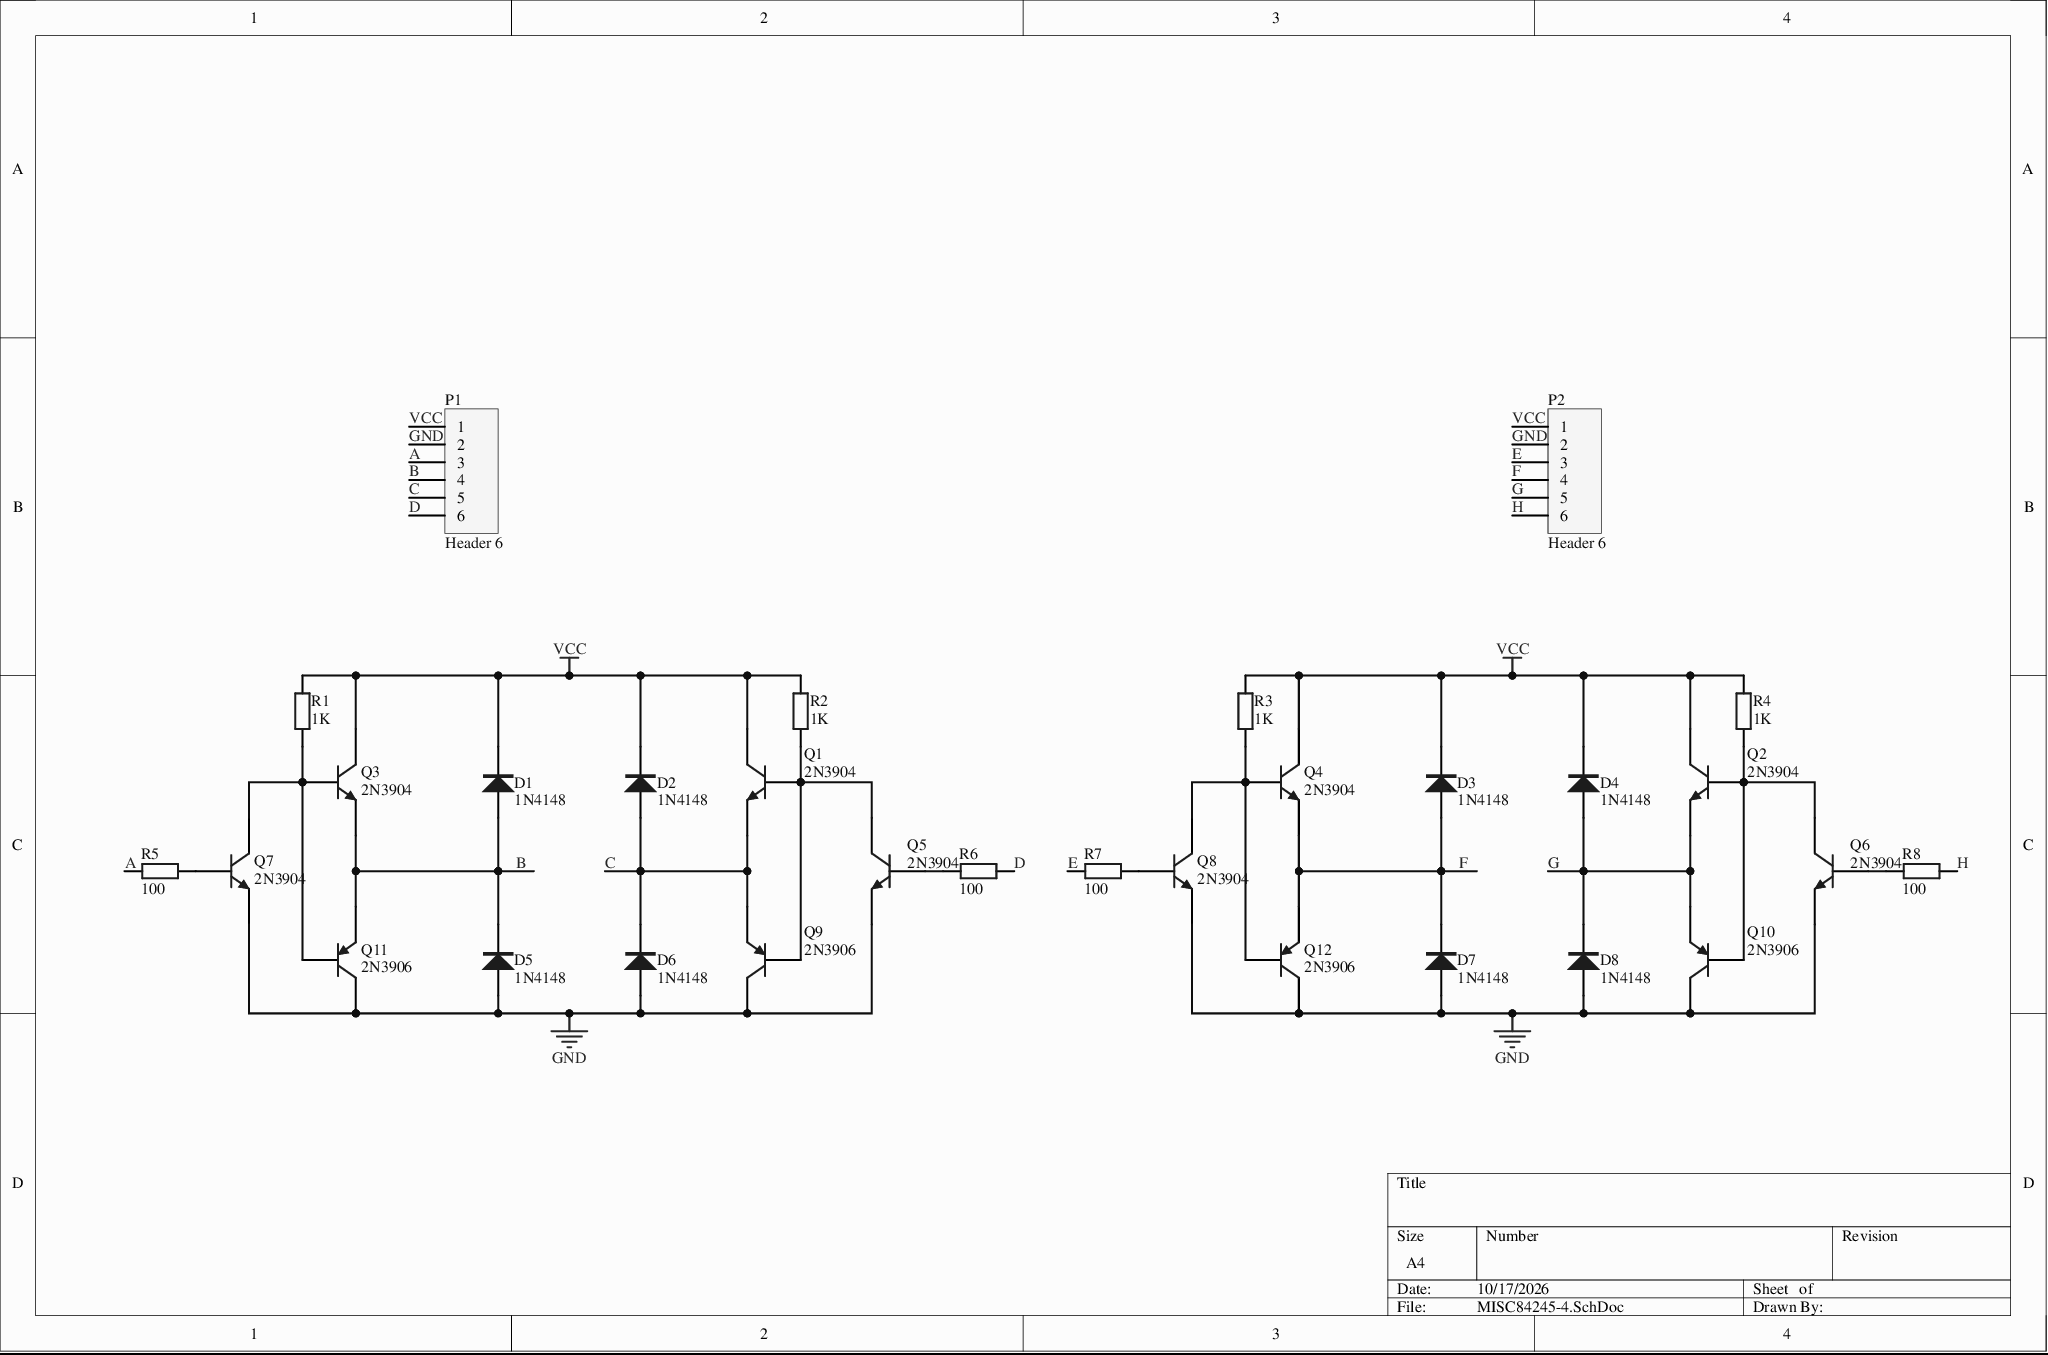
[diagram p0: MISC84245-4.SchDoc]
# Altium project MISC84245-7.PrjPcb
1 sheet, 30 parts. Net scope: global (net labels, ports and power ports of the same name join across sheets).
Board file: MISC84245.PcbDoc

## Sheet MISC84245-4.SchDoc
size A4

### Parts
D1  1N4148  [DO-41]
D2  1N4148  [DO-41]
D3  1N4148  [DO-41]
D4  1N4148  [DO-41]
D5  1N4148  [DO-41]
D6  1N4148  [DO-41]
D7  1N4148  [DO-41]
D8  1N4148  [DO-41]
P1  Header 6  [HDR1X6]
P2  Header 6  [HDR1X6]
Q1  2N3904  [TO-92A]
Q2  2N3904  [TO-92A]
Q3  2N3904  [TO-92A]
Q4  2N3904  [TO-92A]
Q5  2N3904  [TO-92A]
Q6  2N3904  [TO-92A]
Q7  2N3904  [TO-92A]
Q8  2N3904  [TO-92A]
Q9  2N3906  [TO-92A]
Q10  2N3906  [TO-92A]
Q11  2N3906  [TO-92A]
Q12  2N3906  [TO-92A]
R1  1K  [RS 1/4W]
R2  1K  [RS 1/4W]
R3  1K  [RS 1/4W]
R4  1K  [RS 1/4W]
R5  100  [RS 1/4W]
R6  100  [RS 1/4W]
R7  100  [RS 1/4W]
R8  100  [RS 1/4W]

### Nets
GND: D5.1(A) D6.1(A) D7.1(A) D8.1(A) P1.2 P2.2 Q5.1(E) Q6.1(E) Q7.1(E) Q8.1(E) Q9.3(C) Q10.3(C) Q11.3(C) Q12.3(C)
VCC: D1.2(K) D2.2(K) D3.2(K) D4.2(K) P1.1 P2.1 Q1.3(C) Q2.3(C) Q3.3(C) Q4.3(C) R1.2 R2.2 R3.2 R4.2
A: P1.3 R5.2
B: D1.1(A) D5.2(K) P1.4 Q3.1(E) Q11.1(E)
C: D2.1(A) D6.2(K) P1.5 Q1.1(E) Q9.1(E)
D: P1.6 R6.1
E: P2.3 R7.2
F: D3.1(A) D7.2(K) P2.4 Q4.1(E) Q12.1(E)
G: D4.1(A) D8.2(K) P2.5 Q2.1(E) Q10.1(E)
H: P2.6 R8.1
NetQ1_2: Q1.2(B) Q5.3(C) Q9.2(B) R2.1
NetQ2_2: Q2.2(B) Q6.3(C) Q10.2(B) R4.1
NetQ3_2: Q3.2(B) Q7.3(C) Q11.2(B) R1.1
NetQ4_2: Q4.2(B) Q8.3(C) Q12.2(B) R3.1
NetQ5_2: Q5.2(B) R6.2
NetQ6_2: Q6.2(B) R8.2
NetQ7_2: Q7.2(B) R5.1
NetQ8_2: Q8.2(B) R7.1

### Library data of the parts
D1-D8 = 1N4148: Switching diode; BOM名称: High-speed switching diode
P1 P2 = Header 6: Header, 6-Pin; LatestRevisionDate: 17-Jul-2002; LatestRevisionNote: Re-released for DXP Platform.; Publisher: Altium Limited
Q1-Q8 = 2N3904: NPN General Purpose Amplifier; Published: 8-Jun-2000; LatestRevisionDate: 15-Jan-2003; LatestRevisionNote: PCB Footprint 'BCY-W3/D4.7' replaced; DatasheetVersion: 1997; PackageVersion: Sep-1998; PackageReference: TO-92A; PackageDescription: TO, Flat Index; 3 In-Line, Axial Leads; Body Dia. 4.5mm; Leads 0.51 x 0.48 mm (max); ComponentLink1Description: Manufacturer Link; ComponentLink2Description: Datasheet; ComponentLink2URL: http://www.fairchildsemi.com/ds/2N%2F2N3904.pdf; Publisher: Altium Limited
Q9-Q12 = 2N3906: PNP General Purpose Amplifier; Published: 8-Jun-2000; LatestRevisionDate: 15-Jan-2003; LatestRevisionNote: PCB Footprint 'BCY-W3/D4.7' replaced; DatasheetVersion: 1997; PackageVersion: Sep-1998; PackageReference: TO-92A; PackageDescription: TO, Flat Index; 3 In-Line, Axial Leads; Body Dia. 4.5mm; Leads 0.51 x 0.48 mm (max); ComponentLink1Description: Manufacturer Link; ComponentLink2Description: Datasheet; ComponentLink2URL: http://www.fairchildsemi.com/ds/2N%2F2N3906.pdf; Publisher: Altium Limited
R1-R8 = R-S: Color-band resistor; BOM名称: Color-band resistor